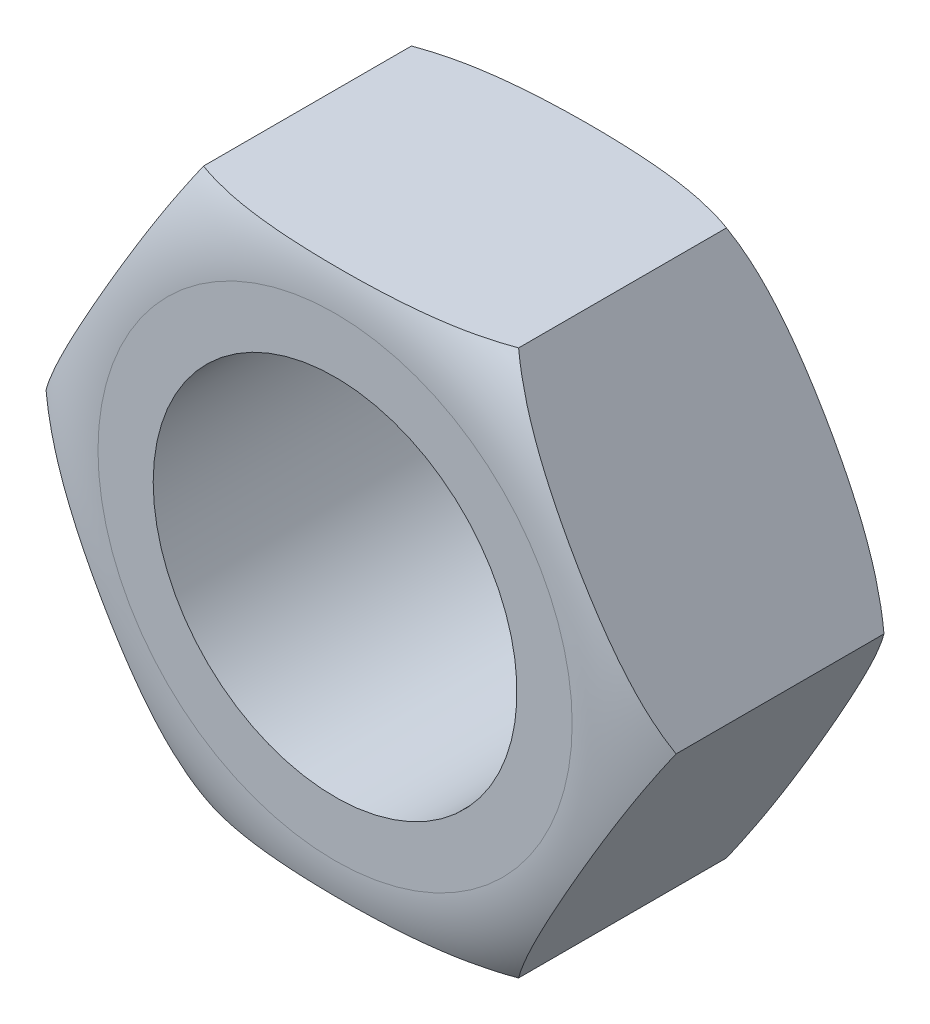
from build123d import *

# Parameters (mm, degrees)
BOSS_EXTRUDE1_DEPTH = 10
SKETCH3_R           = 7
CUT_EXTRUDE1_DEPTH  = 10


with BuildPart() as part:
    # Sketch1 → Boss-Extrude1 (new body)
    with BuildSketch(Plane.XY):
        Polygon((12.124355653, 0), (6.062177826, 10.5), (-6.062177826, 10.5), (-12.124355653, 0), (-6.062177826, -10.5), (6.062177826, -10.5), align=None)
    extrude(amount=BOSS_EXTRUDE1_DEPTH)

    # Sketch2 → Cut-Revolve1 (revolve, cut)
    with BuildSketch(Plane(origin=(0, 0, 0), x_dir=(1, 0, 0), z_dir=(0, 1, 0))):
        with BuildLine():
            Line((-12.124355653, 0), (-12.124355653, -1))
            ThreePointArc((-12.124355653, -1), (-10.705494483, -0.25658351), (-9.124355653, 0))
            Line((-9.124355653, 0), (-12.124355653, 0))
        make_face()
        with BuildLine():
            Line((-12.124355653, -10), (-12.124355653, -9))
            ThreePointArc((-12.124355653, -9), (-10.705494483, -9.74341649), (-9.124355653, -10))
            Line((-9.124355653, -10), (-12.124355653, -10))
        make_face()
    revolve(axis=Axis((0, 0, 0), (0, 0, 1)), mode=Mode.SUBTRACT)

    # Sketch3 → Cut-Extrude1 (cut)
    with BuildSketch(Plane(origin=(0, 0, 0), x_dir=(-1, 0, 0), z_dir=(0, 0, -1))):
        Circle(SKETCH3_R)
    extrude(amount=-CUT_EXTRUDE1_DEPTH, mode=Mode.SUBTRACT)


solid = part.part
